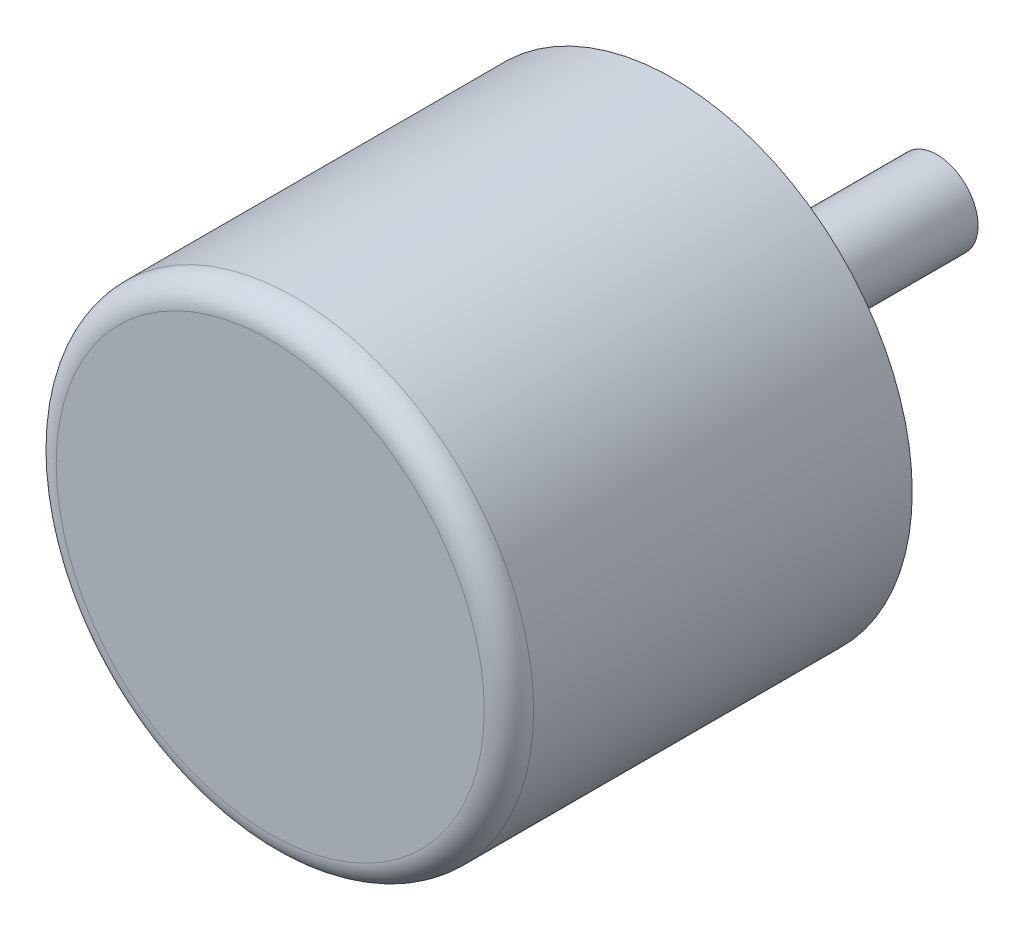
from build123d import *

# Parameters (mm, degrees)
SKETCH_1_R               = 29
EXTRUDE_1_DEPTH          = 24.5
FILLET_1_R               = 3
SKETCH_2_R               = 5
EXTRUDE_2_DEPTH          = 32
PATTERN_CIRCULAR_1_COUNT = 3
SKETCH_5_R               = 18
EXTRUDE_3_DEPTH          = 2.5


with BuildPart() as part:
    # 草图1 → 凸台-拉伸1 (new, symmetric)
    with BuildSketch(Plane.XY):
        Circle(SKETCH_1_R)
    extrude(amount=EXTRUDE_1_DEPTH, both=True)

    # 圆角1
    fillet_1_edges = [part.edges().sort_by_distance(p)[0] for p in [
        (-29, 0, 24.5),
    ]]
    fillet(fillet_1_edges, radius=FILLET_1_R)

    # 草图2 → 凸台-拉伸2 (add)
    with BuildSketch(Plane(origin=(0, 0, -24.5), x_dir=(-1, 0, 0), z_dir=(0, 0, -1))):
        with Locations(Location((0, 0, 0), (0, 0, 180))):
            Circle(SKETCH_2_R)
    extrude(amount=EXTRUDE_2_DEPTH)

    # 草图3 → M3 螺纹孔1 (revolve, cut)
    with BuildSketch(Plane(origin=(-24, 0, -24.5), x_dir=(0, 1, 0), z_dir=(1, 0, 0))):
        Polygon((0, 0), (0, 8.251075774), (1.25, 7.5), (1.25, 0), align=None)
    hole_wizard_m3_1 = revolve(axis=Axis((-24, 0, -30.85), (0, 0, 1)), mode=Mode.SUBTRACT)

    # 阵列(圆周)1: M3 螺纹孔1 ×3 about axis
    pattern_circular_1_axis = Axis((0, 0, 0), (0, 0, 1))
    for i in range(1, PATTERN_CIRCULAR_1_COUNT):
        add(hole_wizard_m3_1.rotate(pattern_circular_1_axis, i * 360 / PATTERN_CIRCULAR_1_COUNT), mode=Mode.SUBTRACT)

    # 草图5 → 凸台-拉伸3 (add)
    with BuildSketch(Plane(origin=(0, 0, -24.5), x_dir=(-1, 0, 0), z_dir=(0, 0, -1))):
        with Locations(Location((0, 0, 0), (0, 0, 180))):
            Circle(SKETCH_5_R)
    extrude(amount=EXTRUDE_3_DEPTH)


solid = part.part
